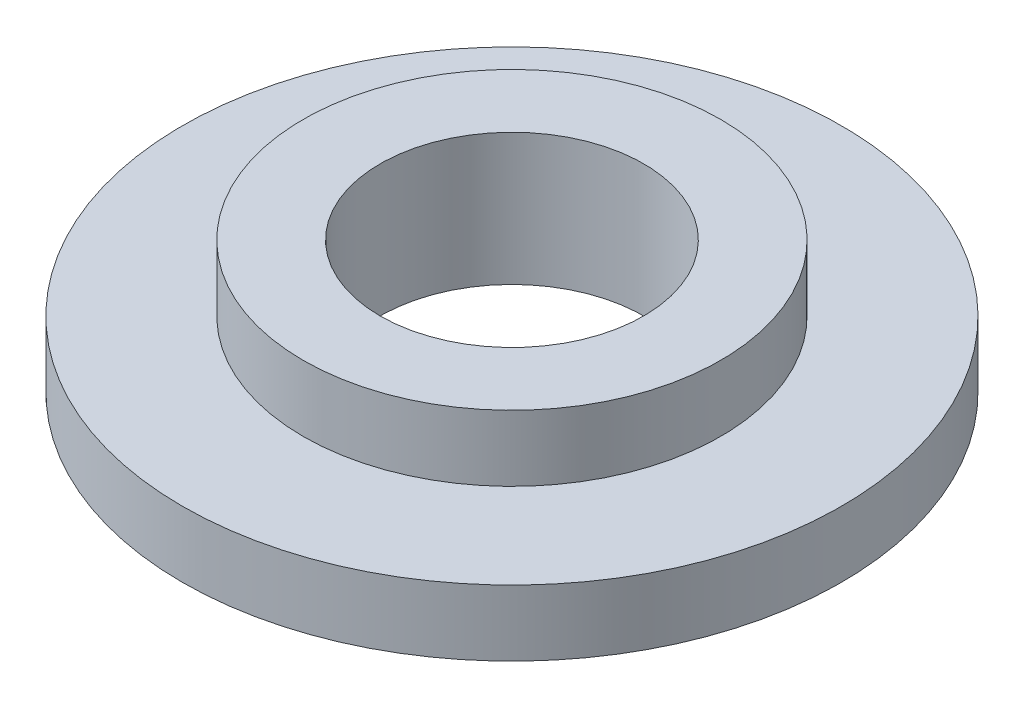
SolidWorks part; units mm, degrees
ref_plane "Front Plane" through (0, 0, 0) normal (0, 0, 1) x (1, 0, 0)
ref_plane "Top Plane" through (0, 0, 0) normal (0, 1, 0) x (1, 0, 0)
ref_plane "Right Plane" through (0, 0, 0) normal (1, 0, 0) x (0, 0, -1)
other "Configuration Table"
sketch "Sketch1" plane through (0, 0, 0) normal (0, 1, 0) x (1, 0, 0)
  circle A0 centre (0, 0) radius 15
  dimension "D1" = 30
extrude "Boss-Extrude1" add sketch "Sketch1" along normal blind 3
sketch "Sketch2" plane through (0, 3, 0) normal (0, 1, 0) x (1, 0, 0)
  circle A0 centre (0, 0) radius 9.5
  dimension "D1" = 19
extrude "Boss-Extrude2" add sketch "Sketch2" along normal blind 3
sketch "Sketch3" plane through (0, 6, 0) normal (0, 1, 0) x (1, 0, 0)
  circle A0 centre (0, 0) radius 6
  dimension "D1" = 12
extrude "Cut-Extrude1" cut sketch "Sketch3" against normal blind 10
